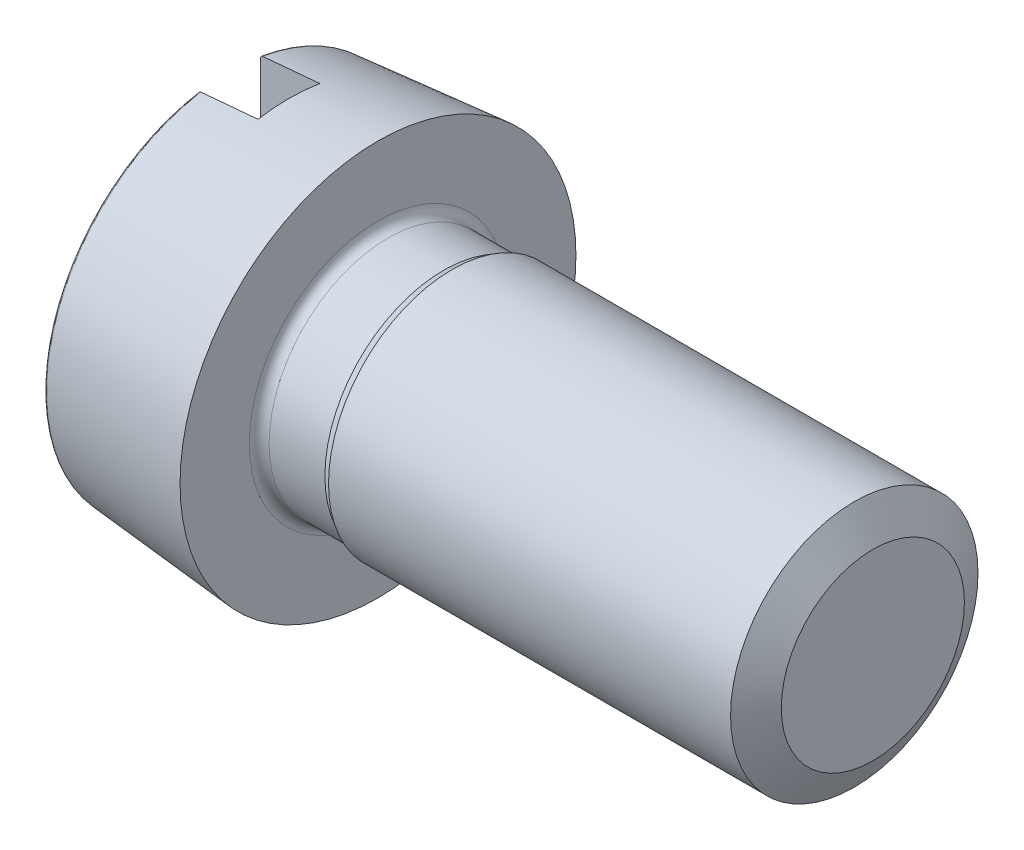
SolidWorks part; units mm, degrees
revolve "基体-旋转" add sketch "草图1" angle 360 about L0
sketch "草图1" plane through (0, 0, 0) normal (0, 0, 1) x (1, 0, 0)
  line L0 (0, 0) -> (26, 0) construction
  line L1 (0, 0) -> (0, 7.3834)
  line L2 (6, 8) -> (0.0913, 7.4831)
  line L3 (6, 8) -> (6, 5.2)
  line L4 (6.4, 4.8) -> (8.6536, 4.8)
  line L5 (8.6536, 4.8) -> (9, 5)
  line L6 (9, 5) -> (26, 5)
  line L7 (26, 5) -> (26, 0)
  line L8 (0, 0) -> (26, 0)
  arc A0 (6.4, 4.8) -> (6, 5.2) centre (6.4, 5.2) cw
  arc A1 (0, 7.3834) -> (0.0913, 7.4831) centre (0.1, 7.3834) cw
cosmetic thread "装饰螺纹线1" parameters "D1"=3.3866, "D2"=1.2
material "4.8级"
ref_plane "前视" through (0, 0, 0) normal (0, 0, 1) x (1, 0, 0)
ref_plane "上视" through (0, 0, 0) normal (0, 1, 0) x (1, 0, 0)
ref_plane "右视" through (0, 0, 0) normal (1, 0, 0) x (0, 0, -1)
sketch "尺寸草图" plane through (0, 0, 0) normal (0, 0, 1) x (1, 0, 0)
  line L0 (0, 0) -> (26, 0)
  point P3 (2.4, 0)
  point P4 (3, 0)
  point P5 (10, 0)
  point P6 (16, 0)
  point P7 (2.5, 0)
  point P8 (3.1989, 0)
  point P9 (3.656, 0)
  point P10 (4.0948, 0)
  point P11 (24.5, 0)
  point P12 (25.6, 0)
  point P13 (6, 0)
sketch "草图2" plane through (0, 0, 0) normal (-1, 0, 0) x (0, 0, 1)
  line L0 (0, 0) -> (0, -1.8809) construction
  line L3 (1.25, 7.9017) -> (1.25, -7.9017)
  line L5 (-1.25, 7.9017) -> (-1.25, -7.9017)
  circle A1 centre (0, 0) radius 8 construction
  arc A2 (1.25, 7.9017) -> (-1.25, 7.9017) centre (0, 0) ccw
  arc A3 (-1.25, -7.9017) -> (1.25, -7.9017) centre (0, 0) ccw
extrude "切除-拉伸1" cut sketch "草图2" against normal blind 2.4
sketch "草图3" plane through (0, 0, 0) normal (0, 1, 0) x (1, 0, 0)
  line L0 (25.25, 5) -> (26.75, 5)
  line L2 (26.75, 5) -> (26, 3.701)
  line L3 (26, 3.701) -> (25.25, 5)
  line L4 (26, -1.6037) -> (26, 3.368) construction
  line L10 (26, -5) -> (26, 5) construction
  line L11 (0, 0) -> (7.2232, 0) construction
revolve "切除-旋转1" cut sketch "草图3" angle 360 about L11
pattern_linear "阵列(线性)1" [suppressed] count 12 along (1, 0, 0)
equation "\"l@草图1\" = \"l@尺寸草图\" "
equation "\"a@草图1\" = \"a@尺寸草图\" "
equation "\"r@草图1\" = \"r@尺寸草图\" "
equation "\"d@草图1\" = \"d@尺寸草图\" "
equation "\"k@草图1\" = \"k@尺寸草图\" "
equation "\"dk@草图1\" = \"dk@尺寸草图\" "
equation "\"n@草图2\" = \"n@尺寸草图\" "
equation "\"t@切除-拉伸1\" = \"t@尺寸草图\" "
equation "\"p@阵列(线性)1\" = \"p@尺寸草图\" "
equation "\"D2@草图3\" = \"p@尺寸草图\" * 0.866"
equation "\"D3@草图3\" = \"d@草图1\" / 2"
equation "\"D1@草图1\" = \"d@草图1\" - \"r@草图1\""
equation "\"D1@阵列(线性)1\" =  ( \"l@草图1\" - \"a@草图1\" )  / \"p@阵列(线性)1\" + 1"
